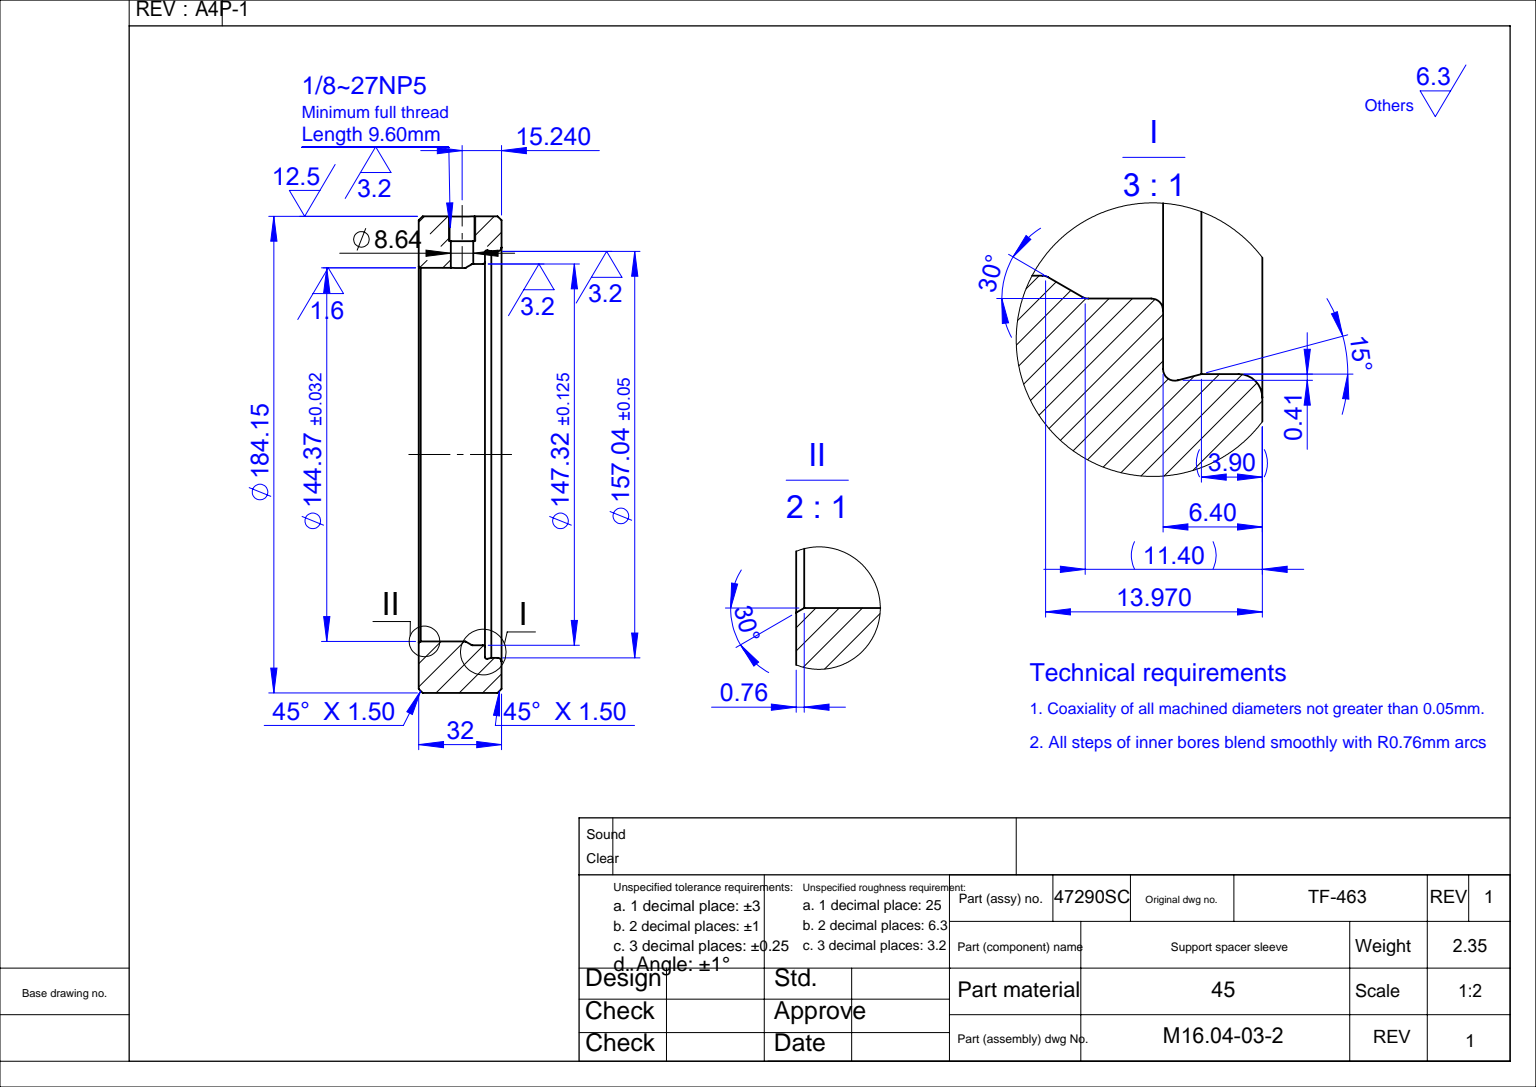
SolidWorks part; units mm, degrees
material "45"
ref_plane "Front Plane" through (0, 0, 0) normal (0, 0, 1) x (1, 0, 0)
ref_plane "Top Plane" through (0, 0, 0) normal (0, 1, 0) x (1, 0, 0)
ref_plane "Right Plane" through (0, 0, 0) normal (1, 0, 0) x (0, 0, -1)
sketch "Sketch1" plane through (0, 0, 0) normal (0, 0, 1) x (1, 0, 0)
  line L0 (-48.0801, 0) -> (53.6066, 0) construction
  line L1 (0, 58.5804) -> (0, -55.2645) construction
  line L2 (0, 92.075) -> (32, 92.075)
  line L3 (32, 92.075) -> (32, 80.044)
  line L4 (30.476, 78.52) -> (28.0759, 78.52)
  line L5 (25.6, 74.422) -> (25.6, 78.1904)
  line L6 (24.838, 73.66) -> (20.7858, 73.66)
  line L7 (20.4048, 73.5579) -> (18.2068, 72.2889)
  line L8 (17.8258, 72.1868) -> (0, 72.1868)
  line L9 (0, 72.1868) -> (0, 92.075)
  line L10 (26.5592, 78.9264) -> (28.0759, 78.52)
  arc A0 (26.5592, 78.9264) -> (25.6, 78.1904) centre (26.362, 78.1904) ccw
  arc A1 (32, 80.044) -> (30.476, 78.52) centre (30.476, 80.044) cw
  arc A2 (18.2068, 72.2889) -> (17.8258, 72.1868) centre (17.8258, 72.9488) cw
  arc A3 (20.7858, 73.66) -> (20.4048, 73.5579) centre (20.7858, 72.898) ccw
  arc A4 (25.6, 74.422) -> (24.838, 73.66) centre (24.838, 74.422) cw
  point P20 (18.03, 72.1868)
  point P23 (20.5817, 73.66)
  dimension "D10" = 1.524
  dimension "D12" = 1.524
  dimension "D14" = 0.762
  dimension "D1" = 184.15
  dimension "D2" = 157.04
  dimension "D3" = 147.32
  dimension "D4" = 144.3736
  dimension "D5" = 32
  dimension "D6" = 6.4
  dimension "D7" = 13.97
  dimension "D8" = 11.4183
  dimension "D9" = 15
  dimension "D11" = 0.4064
  dimension "D13" = 30
revolve "Revolve1" add sketch "Sketch1" angle 360 about L0
chamfer "Chamfer2" distance 0.762 angle 30 1 edges at (0, 0, 72.1868)
chamfer "Chamfer3" distance 1.524 angle 45 2 edges at (32, 0, 92.075) (0, 0, 92.075)
ref_plane "Plane1" through (16, 92.075, 0) normal (0, 1, 0) x (0, 0, -1)
sketch "Sketch2" plane through (16, 92.075, 0) normal (0, 1, 0) x (0, 0, -1)
  line L0 (-90.551, -16) -> (90.551, -16) construction
  line L1 (0, 6.2988) -> (0, -11.6294) construction
  point P0 (0, -0.76)
  dimension "D1" = 15.24
hole_wizard "1/8 NPT Tapped Hole1" positions "3DSketch1" profile "Sketch3" size "1/8" standard "Ansi Inch"
sketch3d "3DSketch1"
  point P0 (16.76, 92.075, 0)
  point P3 (16.76, 92.075, 0)
  point P8 (16.76, 92.075, 0)
sketch "Sketch3" plane through (16.76, 92.075, 0) normal (1, 0, 0) x (0, 0, 1)
  line L0 (0, 0) -> (0, 22.0255)
  line L1 (4.318, 19.431) -> (0, 22.0255)
  line L2 (-4.318, 19.431) -> (0, 22.0255) construction
  line L3 (4.318, 19.431) -> (4.318, 9.652)
  line L4 (4.318, 9.652) -> (4.8264, 9.652)
  line L5 (4.8264, 9.652) -> (4.8264, 0)
  line L6 (-4.8264, 9.652) -> (-4.8264, 0) construction
  line L7 (4.8264, 0) -> (0, 0)
  line L8 (0, -6.35) -> (0, 107.95) construction
  line L11 (-4.318, 9.652) -> (-4.8264, 9.652) construction
  dimension "蹟恇謂郰芛眻噤" = 8.636
  dimension "蹟恇謂郰芛旮僅" = 19.431
  dimension "蹟恇眻噤" = 9.6528
  dimension "蹟恇褒僅" = 0
  dimension "蹟恇旮僅" = 9.652
  dimension "絳芛褒僅" = 118
cosmetic thread "Hole thread 2" parameters "D1"=9.652, "D2"=10.4503
sketch "Sketch4" plane through (0, 0, 0) normal (0, 1, 0) x (1, 0, 0)
  circle A0 centre (16.76, 0) radius 4.318
  arc A1 (18.985, 3.7006) -> (18.985, -3.7006) centre (16.76, 0) ccw construction
extrude "Cut-Extrude1" cut sketch "Sketch4" along normal up to surface (82.423 mm away) up to face at (16.76, 82.423, 4.318)
